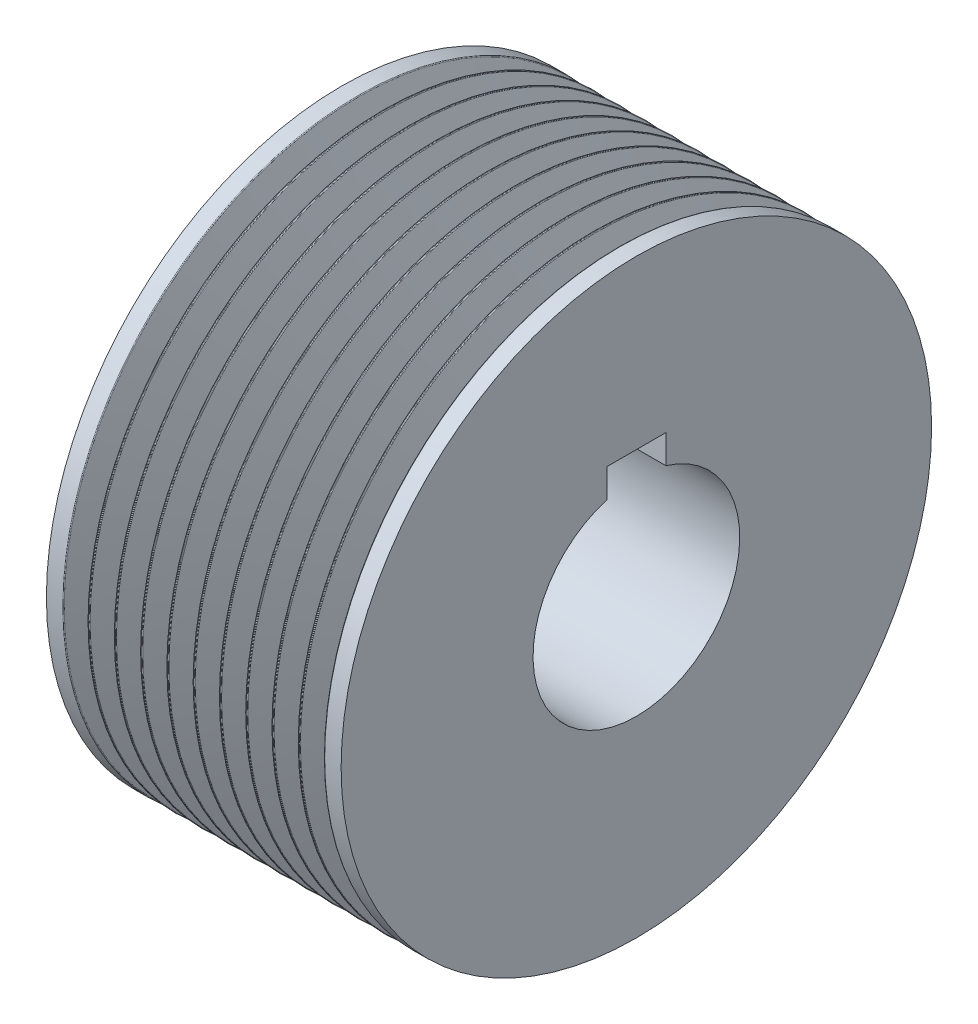
from build123d import *

# Parameters (mm, degrees)
CUT_EXTRUDE1_DEPTH = 98.951033297


with BuildPart() as part:
    # Sketch1 → Revolve1 (revolve)
    with BuildSketch(Plane.XY, mode=Mode.PRIVATE) as revolve1_sk:
        with BuildLine():
            ThreePointArc((-0.02, 0), (-0.090710678, -0.029289322), (-0.12, -0.1))
            Line((-0.12, -0.1), (-1.279429014, -3.285505036))
            ThreePointArc((-1.279429014, -3.285505036), (-1.37095806, -3.404788011), (-1.514352169, -3.45))
            Line((-1.514352169, -3.45), (-1.974352169, -3.45))
            ThreePointArc((-1.974352169, -3.45), (-2.117746278, -3.404788011), (-2.209275325, -3.285505036))
            Line((-2.209275325, -3.285505036), (-3.381152854, -0.065797986))
            ThreePointArc((-3.381152854, -0.065797986), (-3.417764472, -0.018084796), (-3.475122116, 0))
            Line((-3.475122116, 0), (-3.56525059, 0))
            ThreePointArc((-3.56525059, 0), (-3.62251469, -0.018019375), (-3.659141524, -0.065583542))
            Line((-3.659141524, -0.065583542), (-4.839625447, -3.286040922))
            ThreePointArc((-4.839625447, -3.286040922), (-4.931192378, -3.404951088), (-5.074352169, -3.45))
            Line((-5.074352169, -3.45), (-5.534352169, -3.45))
            ThreePointArc((-5.534352169, -3.45), (-5.677746278, -3.404788011), (-5.769275325, -3.285505036))
            Line((-5.769275325, -3.285505036), (-6.941152854, -0.065797986))
            ThreePointArc((-6.941152854, -0.065797986), (-6.977764472, -0.018084796), (-7.035122116, 0))
            Line((-7.035122116, 0), (-7.12525059, 0))
            ThreePointArc((-7.12525059, 0), (-7.18251469, -0.018019375), (-7.219141524, -0.065583542))
            Line((-7.219141524, -0.065583542), (-8.399429014, -3.285505036))
            ThreePointArc((-8.399429014, -3.285505036), (-8.49095806, -3.404788011), (-8.634352169, -3.45))
            Line((-8.634352169, -3.45), (-9.094352169, -3.45))
            ThreePointArc((-9.094352169, -3.45), (-9.237746278, -3.404788011), (-9.329275325, -3.285505036))
            Line((-9.329275325, -3.285505036), (-10.501152854, -0.065797986))
            ThreePointArc((-10.501152854, -0.065797986), (-10.537764472, -0.018084796), (-10.595122116, 0))
            Line((-10.595122116, 0), (-10.68525059, 0))
            ThreePointArc((-10.68525059, 0), (-10.74251469, -0.018019375), (-10.779141524, -0.065583542))
            Line((-10.779141524, -0.065583542), (-11.959429014, -3.285505036))
            ThreePointArc((-11.959429014, -3.285505036), (-12.05095806, -3.404788011), (-12.194352169, -3.45))
            Line((-12.194352169, -3.45), (-12.654352169, -3.45))
            ThreePointArc((-12.654352169, -3.45), (-12.797746278, -3.404788011), (-12.889275325, -3.285505036))
            Line((-12.889275325, -3.285505036), (-14.061152854, -0.065797986))
            ThreePointArc((-14.061152854, -0.065797986), (-14.097764472, -0.018084796), (-14.155122116, 0))
            Line((-14.155122116, 0), (-14.24525059, 0))
            ThreePointArc((-14.24525059, 0), (-14.30251469, -0.018019375), (-14.339141524, -0.065583542))
            Line((-14.339141524, -0.065583542), (-15.519429014, -3.285505036))
            ThreePointArc((-15.519429014, -3.285505036), (-15.61095806, -3.404788011), (-15.754352169, -3.45))
            Line((-15.754352169, -3.45), (-16.214352169, -3.45))
            ThreePointArc((-16.214352169, -3.45), (-16.357746278, -3.404788011), (-16.449275325, -3.285505036))
            Line((-16.449275325, -3.285505036), (-17.621152854, -0.065797986))
            ThreePointArc((-17.621152854, -0.065797986), (-17.657764472, -0.018084796), (-17.715122116, 0))
            Line((-17.715122116, 0), (-17.80525059, 0))
            ThreePointArc((-17.80525059, 0), (-17.86251469, -0.018019375), (-17.899141524, -0.065583542))
            Line((-17.899141524, -0.065583542), (-19.079429014, -3.285505036))
            ThreePointArc((-19.079429014, -3.285505036), (-19.17095806, -3.404788011), (-19.314352169, -3.45))
            Line((-19.314352169, -3.45), (-19.774352169, -3.45))
            ThreePointArc((-19.774352169, -3.45), (-19.917746278, -3.404788011), (-20.009275325, -3.285505036))
            Line((-20.009275325, -3.285505036), (-21.181152854, -0.065797986))
            ThreePointArc((-21.181152854, -0.065797986), (-21.217764472, -0.018084796), (-21.275122116, 0))
            Line((-21.275122116, 0), (-21.36525059, 0))
            ThreePointArc((-21.36525059, 0), (-21.42251469, -0.018019375), (-21.459141524, -0.065583542))
            Line((-21.459141524, -0.065583542), (-22.639429014, -3.285505036))
            ThreePointArc((-22.639429014, -3.285505036), (-22.73095806, -3.404788011), (-22.874352169, -3.45))
            Line((-22.874352169, -3.45), (-23.334352169, -3.45))
            ThreePointArc((-23.334352169, -3.45), (-23.477746278, -3.404788011), (-23.569275325, -3.285505036))
            Line((-23.569275325, -3.285505036), (-24.741152854, -0.065797986))
            ThreePointArc((-24.741152854, -0.065797986), (-24.777764472, -0.018084796), (-24.835122116, 0))
            Line((-24.835122116, 0), (-24.92525059, 0))
            ThreePointArc((-24.92525059, 0), (-24.98251469, -0.018019375), (-25.019141524, -0.065583542))
            Line((-25.019141524, -0.065583542), (-26.199429014, -3.285505036))
            ThreePointArc((-26.199429014, -3.285505036), (-26.29095806, -3.404788011), (-26.434352169, -3.45))
            Line((-26.434352169, -3.45), (-26.894352169, -3.45))
            ThreePointArc((-26.894352169, -3.45), (-27.037746278, -3.404788011), (-27.129275325, -3.285505036))
            Line((-27.129275325, -3.285505036), (-28.301152854, -0.065797986))
            ThreePointArc((-28.301152854, -0.065797986), (-28.337764472, -0.018084796), (-28.395122116, 0))
            Line((-28.395122116, 0), (-28.48525059, 0))
            ThreePointArc((-28.48525059, 0), (-28.54251469, -0.018019375), (-28.579141524, -0.065583542))
            Line((-28.579141524, -0.065583542), (-29.759429014, -3.285505036))
            ThreePointArc((-29.759429014, -3.285505036), (-29.85095806, -3.404788011), (-29.994352169, -3.45))
            Line((-29.994352169, -3.45), (-30.454352169, -3.45))
            ThreePointArc((-30.454352169, -3.45), (-30.597746278, -3.404788011), (-30.689275325, -3.285505036))
            Line((-30.689275325, -3.285505036), (-31.861152854, -0.065797986))
            ThreePointArc((-31.861152854, -0.065797986), (-31.897764472, -0.018084796), (-31.955122116, 0))
            Line((-31.955122116, 0), (-32.04525059, 0))
            ThreePointArc((-32.04525059, 0), (-32.10251469, -0.018019375), (-32.139141524, -0.065583542))
            Line((-32.139141524, -0.065583542), (-33.319429014, -3.285505036))
            ThreePointArc((-33.319429014, -3.285505036), (-33.41095806, -3.404788011), (-33.554352169, -3.45))
            Line((-33.554352169, -3.45), (-34.014352169, -3.45))
            ThreePointArc((-34.014352169, -3.45), (-34.157746278, -3.404788011), (-34.249275325, -3.285505036))
            Line((-34.249275325, -3.285505036), (-35.410070465, -0.096246599))
            ThreePointArc((-35.410070465, -0.096246599), (-35.440629041, -0.027974518), (-35.51, 0))
            Line((-35.51, 0), (-35.515122116, 0))
            Line((-35.515122116, 0), (-35.60525059, 0))
            Line((-35.60525059, 0), (-37.73, 0))
            Line((-37.73, 0), (-37.73, -40))
            Line((-37.73, -40), (2.2, -40))
            Line((2.2, -40), (2.2, 0))
            Line((2.2, 0), (-0.02, 0))
        make_face()
    revolve(revolve1_sk.sketch.rotate(Axis((-37.73, -40, 0), (1, 0, 0)), 180), axis=Axis((-37.73, -40, 0), (1, 0, 0)))

    # Sketch2 → Cut-Extrude1 (cut, through all)
    with BuildSketch(Plane(origin=(2.2, 0, 0), x_dir=(0, 0, -1), z_dir=(1, 0, 0))):
        with BuildLine():
            Line((-4, -22.7), (4, -22.7))
            Line((4, -22.7), (4, -26.583592135))
            ThreePointArc((4, -26.583592135), (0, -54), (-4, -26.583592135))
            Line((-4, -26.583592135), (-4, -22.7))
        make_face()
    extrude(amount=-CUT_EXTRUDE1_DEPTH, mode=Mode.SUBTRACT)


solid = part.part
